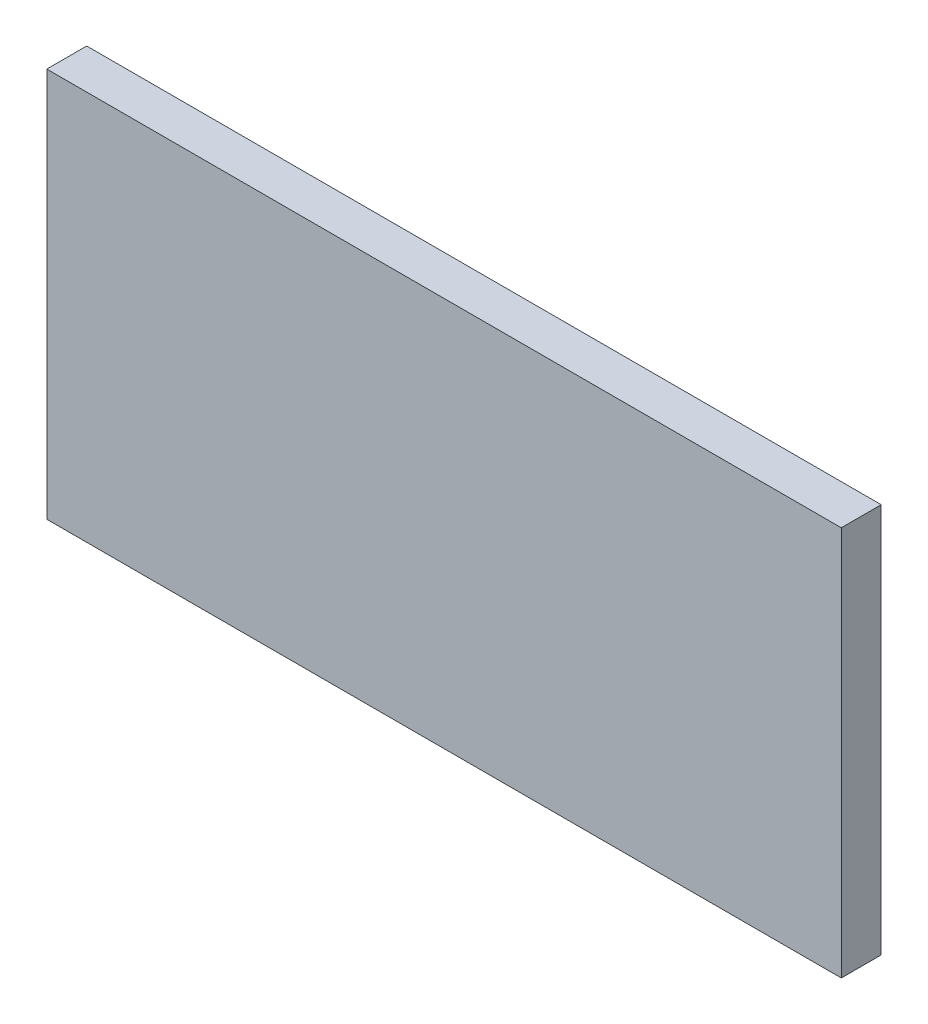
from build123d import *

# Parameters (mm, degrees)
SKETCH_1_W      = 398
SKETCH_1_H      = 195.318610112
EXTRUDE_1_DEPTH = 20


with BuildPart() as part:
    # 草图1 → 凸台-拉伸1 (new body)
    with BuildSketch(Plane.XY):
        with Locations((175, -55.659305056)):
            Rectangle(SKETCH_1_W, SKETCH_1_H)
    extrude(amount=EXTRUDE_1_DEPTH)


solid = part.part
